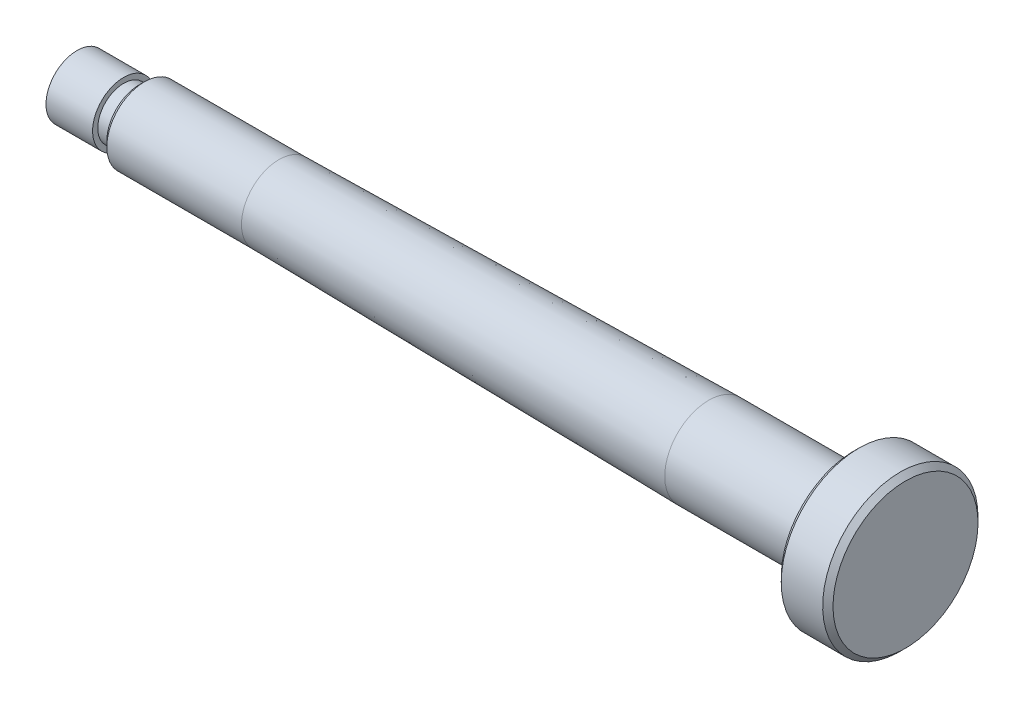
SolidWorks part; units mm, degrees
material "45#"
ref_plane "前视基准面" through (0, 0, 0) normal (0, 0, 1) x (1, 0, 0)
ref_plane "上视基准面" through (0, 0, 0) normal (0, 1, 0) x (1, 0, 0)
ref_plane "右视基准面" through (0, 0, 0) normal (1, 0, 0) x (0, 0, -1)
sketch "草图1" plane through (0, 0, 0) normal (0, 0, 1) x (1, 0, 0)
  line L0 (272.4496, -57.1184) -> (132.4496, -57.1184) construction
  line L1 (272.4496, -10.1184) -> (272.4496, -70.1184) construction
  line L2 (132.4496, -112.1184) -> (132.4496, -46.1184) construction
  line L3 (272.4496, -48.6184) -> (256.4496, -48.6184) construction
  line L5 (134.4496, -49.8684) -> (161.4496, -49.8684)
  line L6 (144.4496, -49.8684) -> (132.4496, -49.8684) construction
  line L7 (161.4496, -49.8684) -> (244.4496, -48.6184)
  line L8 (244.4496, -48.6184) -> (272.4496, -48.6184)
  line L9 (272.4496, -48.6184) -> (272.4496, -42.1184)
  line L10 (272.4496, -42.1184) -> (282.4496, -42.1184)
  line L11 (282.4496, -42.1184) -> (282.4496, -57.1184)
  line L12 (134.4496, -49.8684) -> (134.4496, -52.1184)
  line L13 (134.4496, -52.1184) -> (131.4496, -52.1184)
  line L14 (122.4496, -51.1184) -> (122.4496, -57.1184)
  line L15 (131.4496, -52.1184) -> (131.4496, -51.1184)
  line L16 (131.4496, -51.1184) -> (122.4496, -51.1184)
  line L17 (156.4496, -51.1184) -> (156.4496, -63.1184) construction
  line L18 (282.4496, -57.1184) -> (122.4496, -57.1184)
  dimension "D1" = 8.5
  dimension "D2" = 10
  dimension "D3" = 30
  dimension "D4" = 12
  dimension "D5" = 2
  dimension "D6" = 1
  dimension "D7" = 3
  dimension "D8" = 2
  dimension "D9" = 9
  dimension "D10" = 5
revolve "旋转1" add sketch "草图1" angle 360 about L0
cosmetic thread "装饰螺纹线1" parameters "D2"=10.106
chamfer "倒角1" distance 1 angle 45 3 edges at (134.4496, -49.8684, 0) (282.4496, -42.1184, 0) (272.4496, -42.1184, 0)
